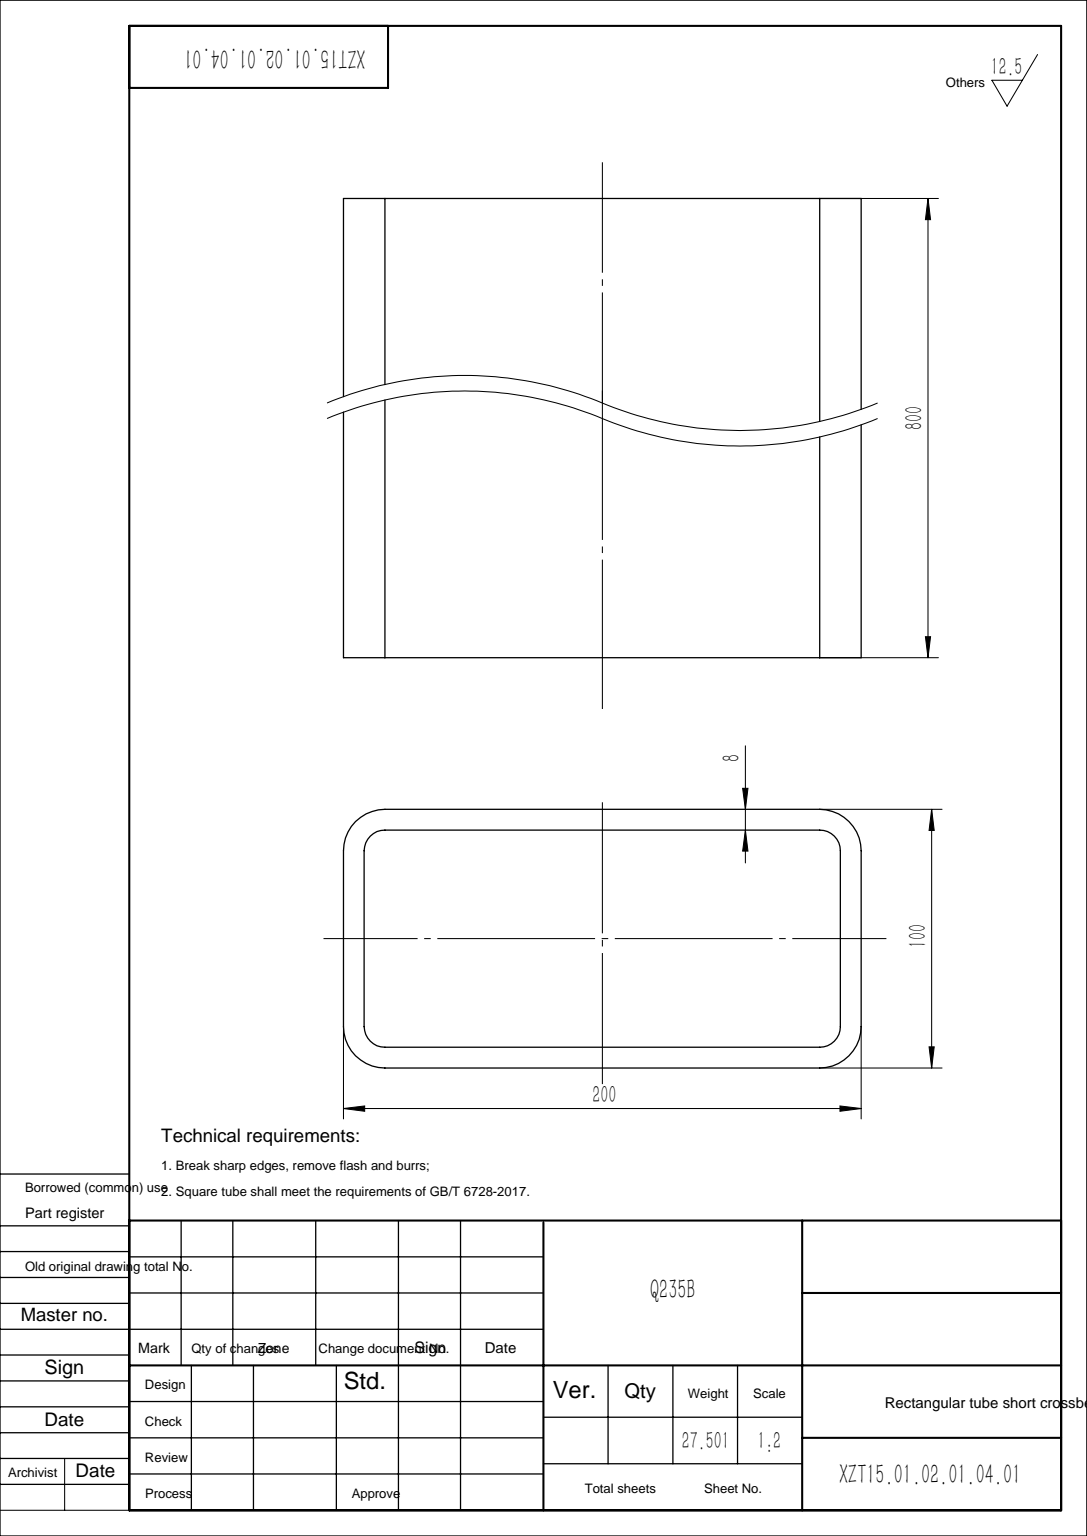
SolidWorks part; units mm, degrees
material "Q235B"
ref_plane "Front Plane" through (0, 0, 0) normal (0, 0, 1) x (1, 0, 0)
ref_plane "Top Plane" through (0, 0, 0) normal (0, 1, 0) x (1, 0, 0)
ref_plane "Right Plane" through (0, 0, 0) normal (1, 0, 0) x (0, 0, -1)
sketch "Sketch1" plane through (0, 0, 0) normal (0, 0, 1) x (1, 0, 0)
  line L0 (0, 0) -> (0, 800)
  dimension "D1" = 800
other "GB/T 6728-2002 rectangular hollow section 200X100X8(2)"
ref_plane "Plane1" through (0, 0, 0) normal (0, 1, 0) x (0, 0, 1)
sketch "Sketch12" plane through (0, 0, 0) normal (0, 1, 0) x (0, 0, 1)
  line L0 (-34, -92) -> (34, -92)
  line L1 (-42, -84) -> (-42, 84)
  line L2 (34, 92) -> (-34, 92)
  line L3 (42, 84) -> (42, -84)
  line L4 (-34, -100) -> (34, -100)
  line L5 (-50, -84) -> (-50, 84)
  line L6 (34, 100) -> (-34, 100)
  line L7 (50, 84) -> (50, -84)
  arc A0 (50, 84) -> (34, 100) centre (34, 84) ccw
  arc A1 (34, -100) -> (50, -84) centre (34, -84) ccw
  arc A2 (-50, -84) -> (-34, -100) centre (-34, -84) ccw
  arc A3 (-34, 100) -> (-50, 84) centre (-34, 84) ccw
  arc A4 (-34, 92) -> (-42, 84) centre (-34, 84) ccw
  arc A5 (42, 84) -> (34, 92) centre (34, 84) ccw
  arc A6 (34, -92) -> (42, -84) centre (34, -84) ccw
  arc A7 (-42, -84) -> (-34, -92) centre (-34, -84) ccw
  point P0 (0, 100)
  point P1 (50, 0)
  point P2 (0, -100)
  point P3 (-50, 0)
  point P4 (-50, 100)
  point P5 (50, 100)
  point P6 (50, -100)
  point P7 (-50, -100)
  point P8 (0, 0)
  point P33 (0, 0)
  dimension "D1" = 16
  dimension "Thickness" = 8
  dimension "V_leg" = 200
  dimension "H_leg" = 100
